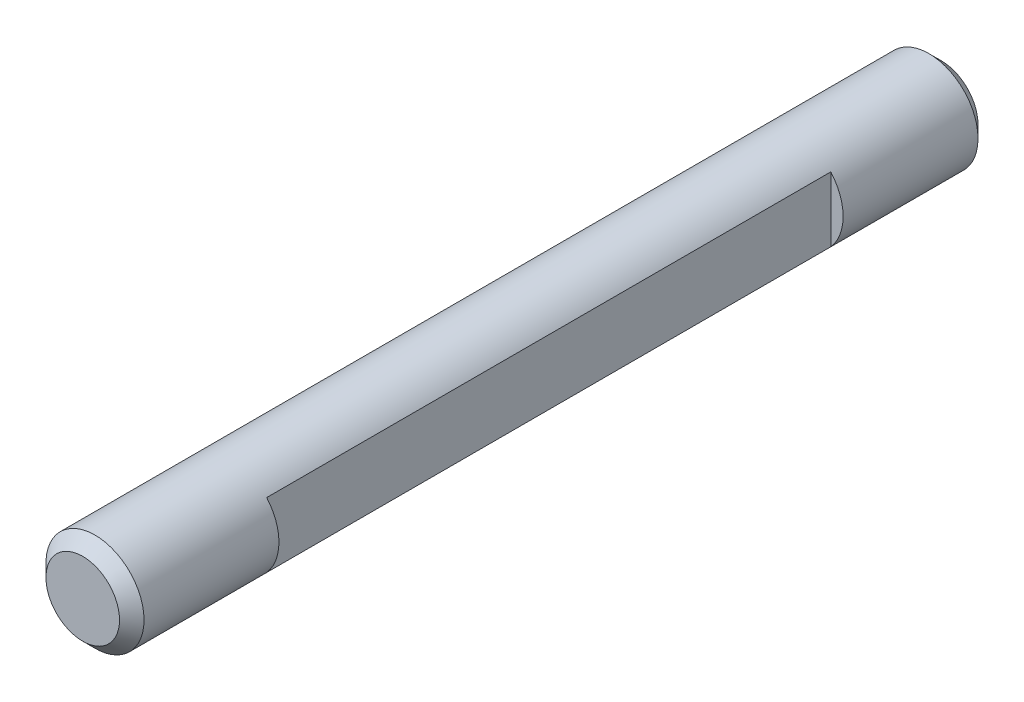
from build123d import *

# Parameters (mm, degrees)
SKETCH1_R           = 2
BOSS_EXTRUDE1_DEPTH = 17.5
CHAMFER1_SIZE       = 0.5
SKETCH2_W           = 1
SKETCH2_H           = 23
CUT_EXTRUDE1_DEPTH  = 5


with BuildPart() as part:
    # Sketch1 → Boss-Extrude1 (new, symmetric)
    with BuildSketch(Plane.XY):
        Circle(SKETCH1_R)
    extrude(amount=BOSS_EXTRUDE1_DEPTH, both=True)

    # Chamfer1
    chamfer1_edges = [part.edges().sort_by_distance(p)[0] for p in [
        (-2, 0, -17.5),
        (-2, 0, 17.5),
    ]]
    chamfer(chamfer1_edges, length=CHAMFER1_SIZE)

    # Sketch2 → Cut-Extrude1 (cut, symmetric)
    with BuildSketch(Plane(origin=(0, 0, 0), x_dir=(1, 0, 0), z_dir=(0, 1, 0))):
        with Locations((2, 0)):
            Rectangle(SKETCH2_W, SKETCH2_H)
    extrude(amount=CUT_EXTRUDE1_DEPTH, both=True, mode=Mode.SUBTRACT)


solid = part.part
